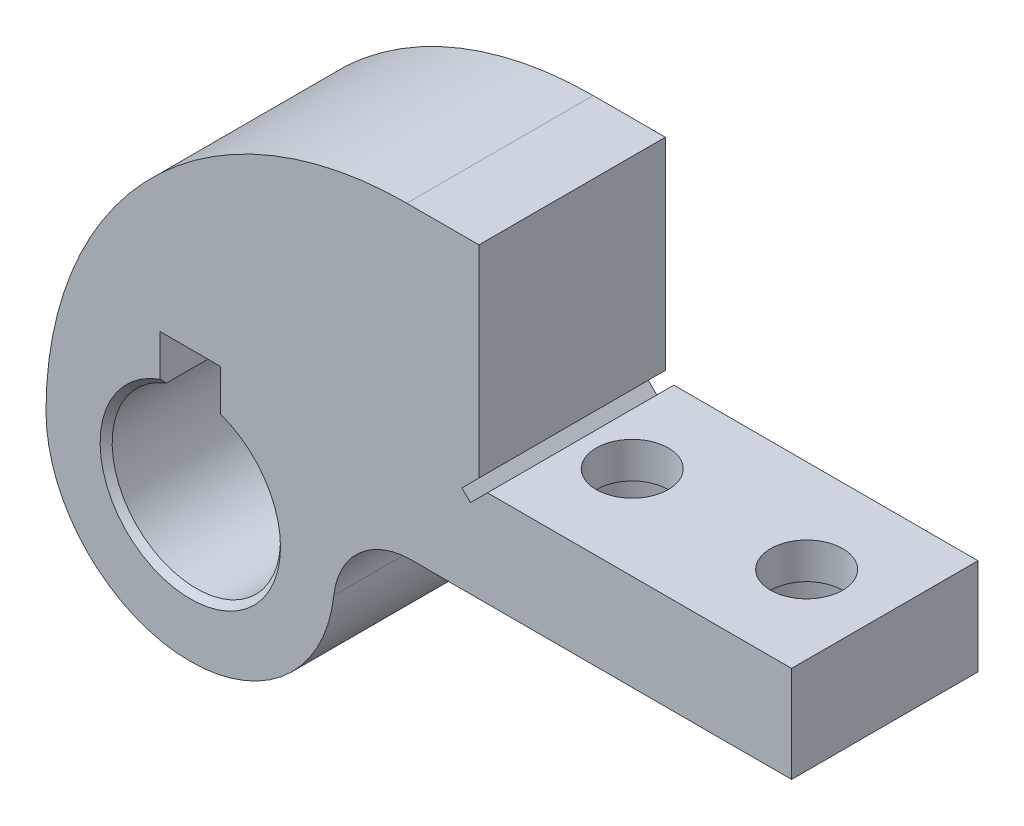
from build123d import *

# Parameters (mm, degrees)
BOSS_EXTRUDE1_DEPTH     = 7.75
CUT_EXTRUDE1_DEPTH      = 57.216656784
CUT_EXTRUDE1_DEPTH_BACK = 57.216656784
SKETCH3_R               = 3
SKETCH4_R               = 5.25
CUT_EXTRUDE2_DEPTH      = 5
CUT_EXTRUDE3_DEPTH      = 61.334484335
CUT_EXTRUDE3_DEPTH_BACK = 61.334484335
CHAMFER2_SIZE           = 0.5


with BuildPart() as part:
    # Sketch2 → Boss-Extrude1 (new, symmetric)
    with BuildSketch(Plane.XY):
        with BuildLine():
            Line((18, 30), (24, 30))
            Line((24, 30), (24, 12.5))
            Line((24, 12.5), (50, 12.5))
            Line((50, 12.5), (50, 4.5))
            Line((50, 4.5), (18.391574158, 4.5))
            ThreePointArc((18.391574158, 4.5), (14.050927176, 2.838262476), (11.929669724, -1.297297297))
            ThreePointArc((11.929669724, -1.297297297), (-0.649601152, -11.982404531), (-12, 0))
            ThreePointArc((-12, 0), (-3.213203436, 21.213203436), (18, 30))
        make_face()
        with BuildLine():
            Line((-2.5, 6.538348415), (-2.5, 10.5))
            Line((-2.5, 10.5), (2.5, 10.5))
            Line((2.5, 10.5), (2.5, 6.538348415))
            ThreePointArc((2.5, 6.538348415), (0, -7), (-2.5, 6.538348415))
        make_face(mode=Mode.SUBTRACT)
    extrude(amount=BOSS_EXTRUDE1_DEPTH, both=True)

    # Sketch3 → Cut-Extrude1 (cut, two sides: drawn at the far end of the back side and taken through both)
    with BuildSketch(Plane(origin=(0, 12.5, 0), x_dir=(1, 0, 0), z_dir=(0, 1, 0)).offset(-CUT_EXTRUDE1_DEPTH_BACK)):
        with Locations(Location((29, 0, 0), (0, 0, 180))):
            Circle(SKETCH3_R)
        with Locations(Location((43.5, 0, 0), (0, 0, 180))):
            Circle(SKETCH3_R)
    extrude(amount=CUT_EXTRUDE1_DEPTH + CUT_EXTRUDE1_DEPTH_BACK, mode=Mode.SUBTRACT)

    # Sketch4 → Cut-Extrude2 (cut)
    with BuildSketch(Plane.XZ.offset(-4.5)):
        with Locations((29, 0)):
            Circle(SKETCH4_R)
        with Locations((43.5, 0)):
            Circle(SKETCH4_R)
    extrude(amount=-CUT_EXTRUDE2_DEPTH, mode=Mode.SUBTRACT)

    # Sketch5 → Cut-Extrude3 (cut, two sides: drawn at the far end of the back side and taken through both)
    with BuildSketch(Plane.XY.offset(7.75).offset(-CUT_EXTRUDE3_DEPTH_BACK)):
        Polygon((24, 13.207106781), (22.585786438, 11.792893219), (23.292893219, 11.085786438), (24.707106781, 12.5), align=None)
    extrude(amount=CUT_EXTRUDE3_DEPTH + CUT_EXTRUDE3_DEPTH_BACK, mode=Mode.SUBTRACT)

    # Chamfer2
    chamfer2_edges = [part.edges().sort_by_distance(p)[0] for p in [
        (0, -7, -7.75),
        (0, -7, 7.75),
    ]]
    chamfer(chamfer2_edges, length=CHAMFER2_SIZE)


solid = part.part
